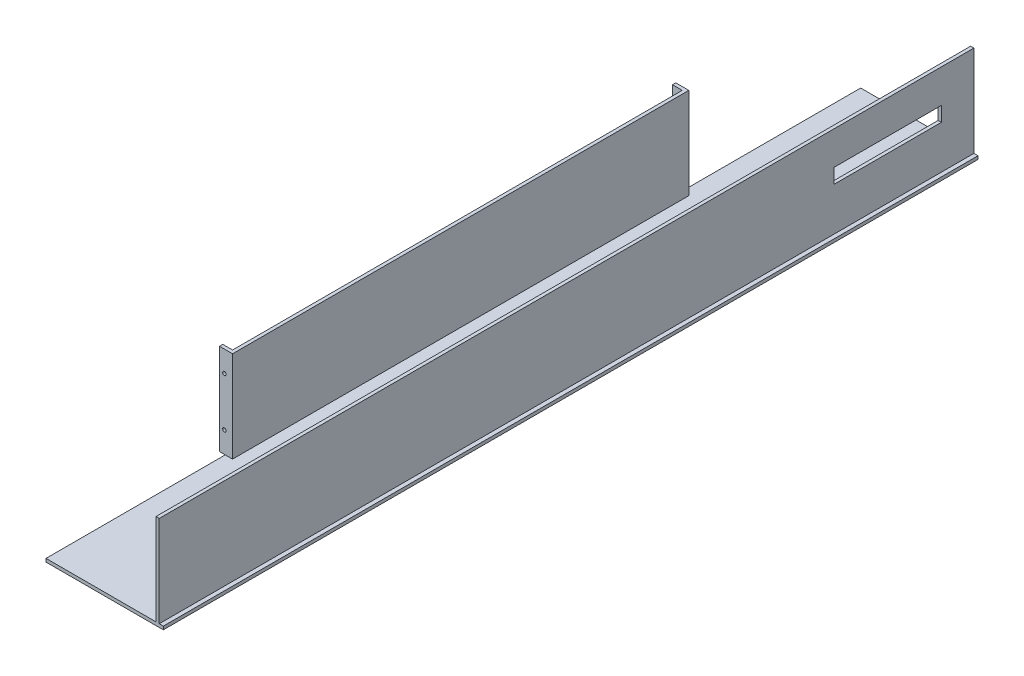
from build123d import *

# Parameters (mm, degrees)
BOSS_EXTRUDE1_DEPTH = 5000
CUT_EXTRUDE1_REACH  = 5083.282
SKETCH2_W           = 660
SKETCH2_H           = 90
SKETCH3_W           = 1100
SKETCH3_H           = 560
CUT_EXTRUDE2_DEPTH  = 20
SKETCH4_W           = 20
SKETCH4_H           = 560
BOSS_EXTRUDE2_DEPTH = 60
SKETCH5_R           = 11
CUT_EXTRUDE3_DEPTH  = 3963.628546811


with BuildPart() as part:
    # Sketch1 → Boss-Extrude1 (new body)
    with BuildSketch(Plane.XY):
        Polygon((360, 0), (-360, 0), (-360, 20), (-335, 20), (-335, 580), (-315, 580), (-315, 20), (315, 20), (315, 580), (335, 580), (335, 20), (360, 20), align=None)
    extrude(amount=BOSS_EXTRUDE1_DEPTH)

    # Sketch2 → Cut-Extrude1 (cut, up to next)
    with BuildSketch(Plane(origin=(335, 0, 0), x_dir=(0, 0, -1), z_dir=(1, 0, 0)), mode=Mode.PRIVATE) as cut_extrude1_sk1:
        with Locations((-530, 330)):
            Rectangle(SKETCH2_W, SKETCH2_H)
    cut_extrude1_tool1 = extrude(cut_extrude1_sk1.sketch, amount=-CUT_EXTRUDE1_REACH, mode=Mode.PRIVATE) & part.part
    add(cut_extrude1_tool1.solids().sort_by_distance((335, 330, 530))[0], mode=Mode.SUBTRACT)

    # Sketch3 → Cut-Extrude2 (cut)
    with BuildSketch(Plane.ZY.offset(335)):
        with Locations((4450, 300)):
            Rectangle(SKETCH3_W, SKETCH3_H)
        with Locations((550, 300)):
            Rectangle(SKETCH3_W, SKETCH3_H)
    extrude(amount=-CUT_EXTRUDE2_DEPTH, mode=Mode.SUBTRACT)

    # Sketch4 → Boss-Extrude2 (add)
    with BuildSketch(Plane.ZY.offset(335)):
        with Locations((1110, 300)):
            Rectangle(SKETCH4_W, SKETCH4_H)
        with Locations((3890, 300)):
            Rectangle(SKETCH4_W, SKETCH4_H)
    extrude(amount=BOSS_EXTRUDE2_DEPTH)

    # Sketch5 → Cut-Extrude3 (cut, through all)
    with BuildSketch(Plane.XY.offset(3900)):
        with Locations((-365, 450)):
            Circle(SKETCH5_R)
        with Locations((-365, 150)):
            Circle(SKETCH5_R)
    extrude(amount=-CUT_EXTRUDE3_DEPTH, mode=Mode.SUBTRACT)


solid = part.part
